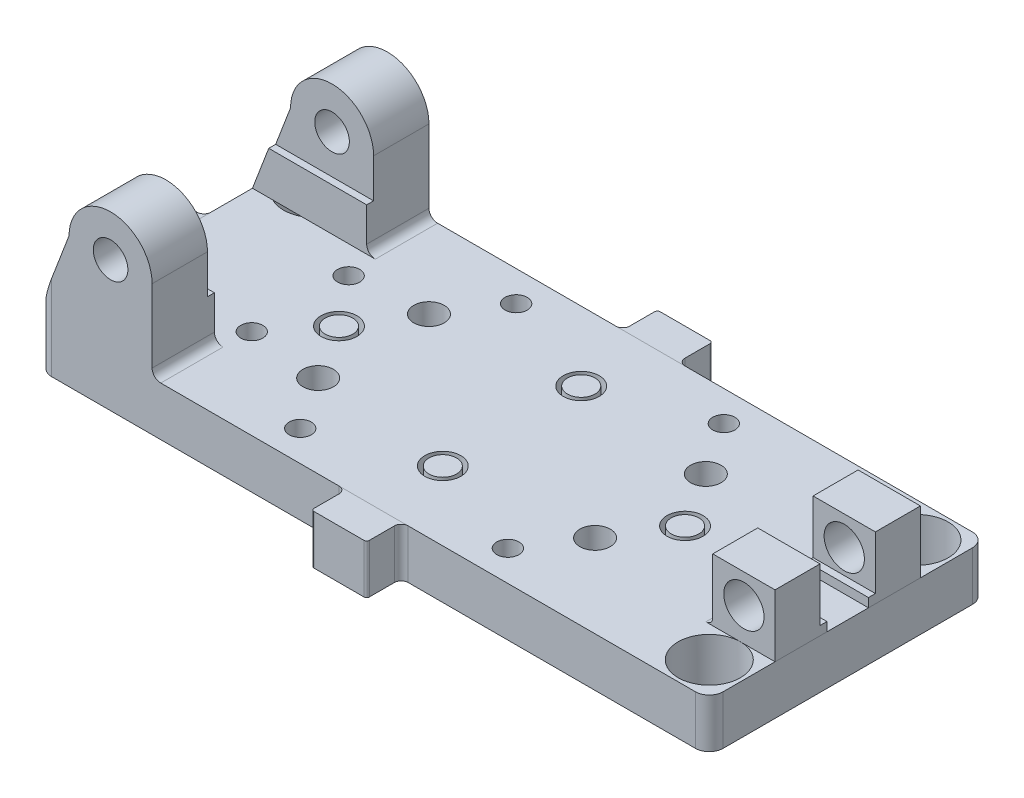
SolidWorks part; units mm, degrees
ref_plane "Front Plane" through (0, 0, 0) normal (0, 0, 1) x (1, 0, 0)
ref_plane "Top Plane" through (0, 0, 0) normal (0, 1, 0) x (1, 0, 0)
ref_plane "Right Plane" through (0, 0, 0) normal (1, 0, 0) x (0, 0, -1)
sketch "Sketch1" plane through (0, 0, 0) normal (0, 0, 1) x (1, 0, 0)
  line L1 (-242.5018, -17.7203) -> (242.5018, -17.7203)
  line L2 (-242.5018, -17.7203) -> (-242.5018, 17.7203)
  line L3 (-153.7539, 17.7203) -> (242.5018, 17.7203)
  line L4 (242.5018, -17.7203) -> (242.5018, 17.7203)
  line L5 (-242.5018, -17.7203) -> (242.5018, 17.7203) construction
  line L6 (-242.5018, 17.7203) -> (242.5018, -17.7203) construction
  line L7 (-242.5018, 17.7203) -> (-220, 76.7203)
  line L8 (-242.5018, 17.7203) -> (-242.5018, -17.2797)
  line L11 (-198.3931, 46.7203) -> (64.8284, 46.7203) construction
  line L12 (-215.3911, 60.7425) -> (-231.7992, 17.7203)
  line L13 (0, 132.5702) -> (0, -92.6193) construction
  line L14 (-231.7992, 17.7203) -> (-231.7992, -17.7203)
  line L15 (-308.8931, 76.7203) -> (-63.6587, 76.7203) construction
  line L16 (-160, 76.7203) -> (-160, 23.9664)
  arc A0 (-160, 76.7203) -> (-215.3911, 60.7425) centre (-190, 76.7203) ccw
  arc A1 (-153.7539, 17.7203) -> (-160, 23.9664) centre (-153.7539, 23.9664) cw
  circle A2 centre (-190, 76.7203) radius 12.5
  point P0 (0, 0)
  point P16 (-223.5952, 39.2314)
  dimension "D1" = 6.2461
  dimension "D2" = 25
  dimension "D6" = 160
  dimension "D4" = 60
  dimension "D7" = 30
  dimension "D8" = 10
extrude "Boss-Extrude1" add sketch "Sketch1" along normal mid plane 200 contours L3 A1 L16 A0 L12 L14 L1 L4 A2 | A0 L7 L2 L1 L14 L12
sketch "Sketch2" plane through (0, 0, 0) normal (1, 0, 0) x (0, 0, -1)
  line L0 (-60, 106.7203) -> (-60, 48.5846)
  line L1 (100, 106.7203) -> (-100, 106.7203) construction
  line L3 (0, 123.1038) -> (0, -40.2879) construction
  line L4 (-60, 48.5846) -> (-55, 48.5846)
  line L5 (-55, 48.5846) -> (-55, 17.7203)
  line L6 (-100, 17.7203) -> (100, 17.7203) construction
  line L8 (-55, 17.7203) -> (55, 17.7203)
  line L9 (-100, 17.7203) -> (100, 17.7203) construction
  line L10 (55, 48.5846) -> (55, 17.7203)
  line L11 (60, 48.5846) -> (55, 48.5846)
  line L12 (60, 106.7203) -> (60, 48.5846)
  line L13 (-60, 106.7203) -> (60, 106.7203)
  point P20 (0, 17.7203)
  dimension "D1" = 60
  dimension "D2" = 5
extrude "Cut-Extrude1" cut sketch "Sketch2" against normal through all both and the other way through all
sketch "Sketch3" plane through (0, 0, 0) normal (0, 0, 1) x (1, 0, 0)
  line L1 (242.5018, 17.7203) -> (192.5018, 17.7203)
  line L2 (242.5018, 17.7203) -> (242.5018, 62.7203)
  line L3 (242.5018, 62.7203) -> (197.5018, 62.7203)
  line L4 (197.5018, 22.7203) -> (197.5018, 62.7203)
  circle A0 centre (220.0018, 41.7203) radius 14.5539
  arc A1 (197.5018, 22.7203) -> (192.5018, 17.7203) centre (192.5018, 22.7203) cw
  dimension "D2" = 21
  dimension "D1" = 5
  dimension "D3" = 45
  dimension "D4" = 22.5
extrude "Boss-Extrude2" add sketch "Sketch3" along normal mid plane 105 separate body
sketch "Sketch4" plane through (0, 0, 0) normal (1, 0, 0) x (0, 0, -1)
  line L0 (0, 125.7076) -> (0, -36.7076) construction
  line L1 (-52.5, 62.7203) -> (52.5, 62.7203) construction
  line L3 (-20, 62.7203) -> (-20, 24.1574)
  line L4 (-20, 24.1574) -> (-15, 24.1574)
  line L7 (-15, 24.1574) -> (-15, 17.7203)
  line L8 (-100, 17.7203) -> (100, 17.7203) construction
  line L9 (-15, 17.7203) -> (15, 17.7203)
  line L10 (15, 24.1574) -> (15, 17.7203)
  line L11 (20, 24.1574) -> (15, 24.1574)
  line L12 (20, 62.7203) -> (20, 24.1574)
  line L13 (-20, 62.7203) -> (20, 62.7203)
  point P17 (0, 17.7203)
  dimension "D2" = 15
  dimension "D3" = 20
extrude "Cut-Extrude3" cut sketch "Sketch4" against normal through all both and the other way through all
sketch "Sketch5" plane through (0, 0, 0) normal (0, 1, 0) x (1, 0, 0)
  line L0 (0, 190.6156) -> (0, -154.3078) construction
  line L1 (-153.7539, 100) -> (242.5018, 100) construction
  line L2 (-20.5218, 100) -> (0, 100)
  line L3 (-20.5218, 100) -> (-20.5218, 125)
  line L4 (-20.5218, 125) -> (0, 125)
  line L5 (0, 100) -> (0, 125)
  line L6 (-328.3481, 0) -> (274.6758, 0) construction
  circle A0 centre (-153, 35) radius 8
  circle A1 centre (-153, -35) radius 8
  circle A2 centre (-125, 0) radius 13
  circle A3 centre (-100, 40) radius 11
  circle A4 centre (-100, -40) radius 11
  circle A5 centre (0, 50) radius 13
  circle A6 centre (0, -50) radius 13
  circle A7 centre (-125, 0) radius 10
  circle A8 centre (0, 50) radius 10
  circle A9 centre (0, -50) radius 10
  circle A10 centre (75, -78) radius 8
  circle A11 centre (100, -40) radius 11
  circle A12 centre (-75, 78) radius 8
  circle A13 centre (-75, -78) radius 8
  circle A14 centre (125, 0) radius 10
  circle A15 centre (125, 0) radius 13
  circle A16 centre (100, 40) radius 11
  circle A17 centre (75, 78) radius 8
  dimension "D2" = 70
  dimension "D7" = 75
  dimension "D11" = 16
  dimension "D12" = 16
  dimension "D15" = 16
  dimension "D16" = 16
  dimension "D19" = 22
  dimension "D20" = 22
  dimension "D21" = 26
  dimension "D22" = 20
  dimension "D23" = 26
  dimension "D24" = 26
  dimension "D25" = 20
  dimension "D26" = 20
  dimension "D1" = 25
  dimension "D3" = 35
  dimension "D4" = 125
  dimension "D5" = 53
  dimension "D6" = 53
  dimension "D8" = 75
  dimension "D9" = 100
  dimension "D10" = 50
  dimension "D13" = 156
  dimension "D14" = 78
  dimension "D17" = 80
  dimension "D18" = 40
  dimension "D27" = 100
extrude "Cut-Extrude4" cut sketch "Sketch5" against normal through all both and the other way through all
sketch "Sketch6" plane through (0, 0, 0) normal (0, 1, 0) x (1, 0, 0)
  line L0 (0, 188.2477) -> (0, -180.3547) construction
  line L1 (-295.9869, 0) -> (325.9802, 0) construction
  line L3 (-247.5018, 20) -> (-265.5018, 20)
  line L4 (-242.5018, 25) -> (-242.5018, -25)
  line L6 (-267.5018, 18) -> (-267.5018, -18)
  line L8 (25, 100) -> (-25, 100)
  line L9 (20, -105) -> (20, -123)
  line L10 (18, 125) -> (-18, 125)
  line L11 (-20, 105) -> (-20, 123)
  line L12 (-247.5018, -20) -> (-265.5018, -20)
  line L14 (20, 105) -> (20, 123)
  line L15 (-20, -105) -> (-20, -123)
  line L16 (18, -125) -> (-18, -125)
  line L17 (25, -100) -> (-25, -100)
  arc A0 (-265.5018, 20) -> (-267.5018, 18) centre (-265.5018, 18) ccw
  arc A1 (-242.5018, 25) -> (-247.5018, 20) centre (-247.5018, 25) cw
  arc A2 (-242.5018, -25) -> (-247.5018, -20) centre (-247.5018, -25) ccw
  arc A3 (-265.5018, -20) -> (-267.5018, -18) centre (-265.5018, -18) cw
  arc A4 (-18, 125) -> (-20, 123) centre (-18, 123) ccw
  arc A5 (-25, 100) -> (-20, 105) centre (-25, 105) ccw
  arc A6 (25, 100) -> (20, 105) centre (25, 105) cw
  arc A7 (18, 125) -> (20, 123) centre (18, 123) cw
  arc A8 (18, -125) -> (20, -123) centre (18, -123) ccw
  arc A9 (25, -100) -> (20, -105) centre (25, -105) ccw
  arc A10 (-25, -100) -> (-20, -105) centre (-25, -105) cw
  arc A11 (-18, -125) -> (-20, -123) centre (-18, -123) cw
  point P7 (-267.5018, -20)
  point P13 (-267.5018, 20)
  point P29 (-267.5018, 0)
  point P30 (-242.5018, 0)
  point P34 (-20, 125)
  point P43 (20, 125)
  point P54 (20, -125)
  point P55 (-20, -125)
  dimension "D3" = 2
  dimension "D4" = 5
  dimension "D7" = 2
  dimension "D5" = 5
  dimension "D1" = 25
  dimension "D2" = 20
extrude "Boss-Extrude5" add sketch "Sketch6" along normal up to vertex (17.7203 mm away) and the other way up to vertex (17.7203 mm away) separate body
sketch "Sketch7" plane through (0, 0, 0) normal (0, 1, 0) x (1, 0, 0)
  line L0 (-402.5923, 0) -> (277.9943, 0) construction
  line L1 (0, -186.731) -> (0, 202.9684) construction
  line L2 (242.5018, -100) -> (242.5018, 100) construction
  line L4 (-153.7539, -100) -> (242.5018, -100) construction
  circle A0 centre (217.5018, -75) radius 22.5
  circle A1 centre (217.5018, 75) radius 22.5
  circle A2 centre (-217.5018, 75) radius 22.5
  circle A3 centre (-217.5018, -75) radius 22.5
  dimension "D1" = 25
  dimension "D2" = 45
  dimension "D3" = 25
extrude "Cut-Extrude5" cut sketch "Sketch7" against normal through all and the other way up to surface (17.7203 mm away) other way up to face at (67, 17.7203, 78)
fillet "Fillet11" radius 10 4 edges at (-242.5018, 0, -100) (-242.5018, 0, 100) (242.5018, 0, 100) (242.5018, 0, -100)
